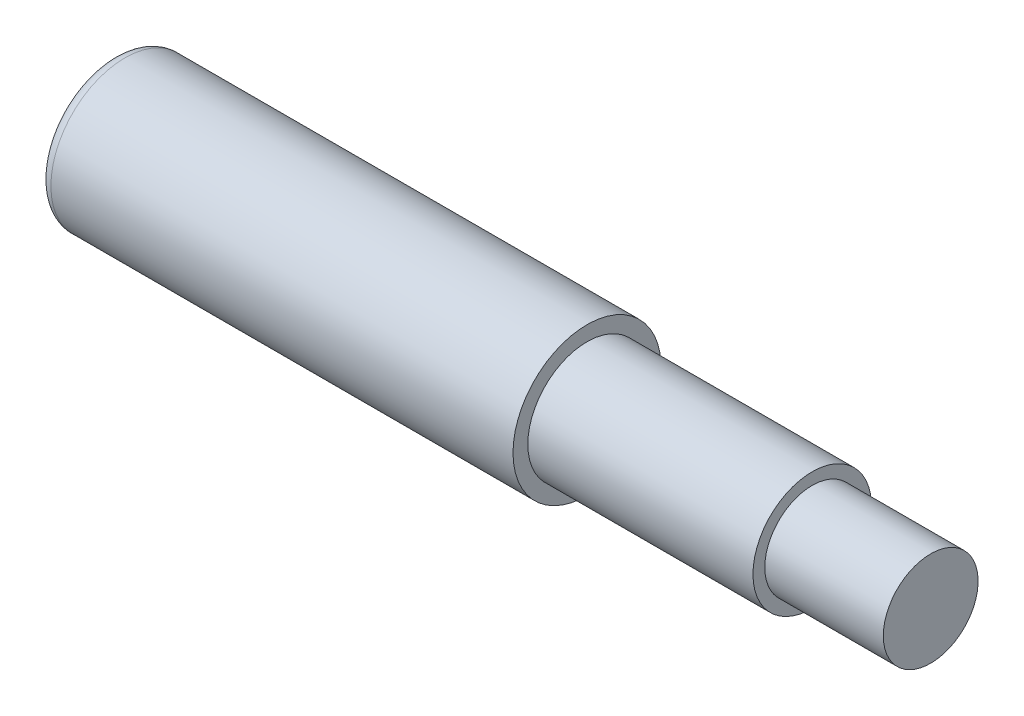
from build123d import *

# Parameters (mm, degrees)
FILLET1_R = 2


with BuildPart() as part:
    # Sketch3 → Revolve1 (revolve)
    with BuildSketch(Plane.XY, mode=Mode.PRIVATE) as revolve1_sk:
        Polygon((0, 0), (0, 12.5), (80, 12.5), (80, 10), (118, 10), (118, 8), (138, 8), (138, 0), align=None)
    revolve(revolve1_sk.sketch.rotate(Axis((0, 0, 0), (1, 0, 0)), 90), axis=Axis((0, 0, 0), (1, 0, 0)))

    # Fillet1
    fillet1_edges = [part.edges().sort_by_distance(p)[0] for p in [
        (0, 0, -12.5),
    ]]
    fillet(fillet1_edges, radius=FILLET1_R)


solid = part.part
